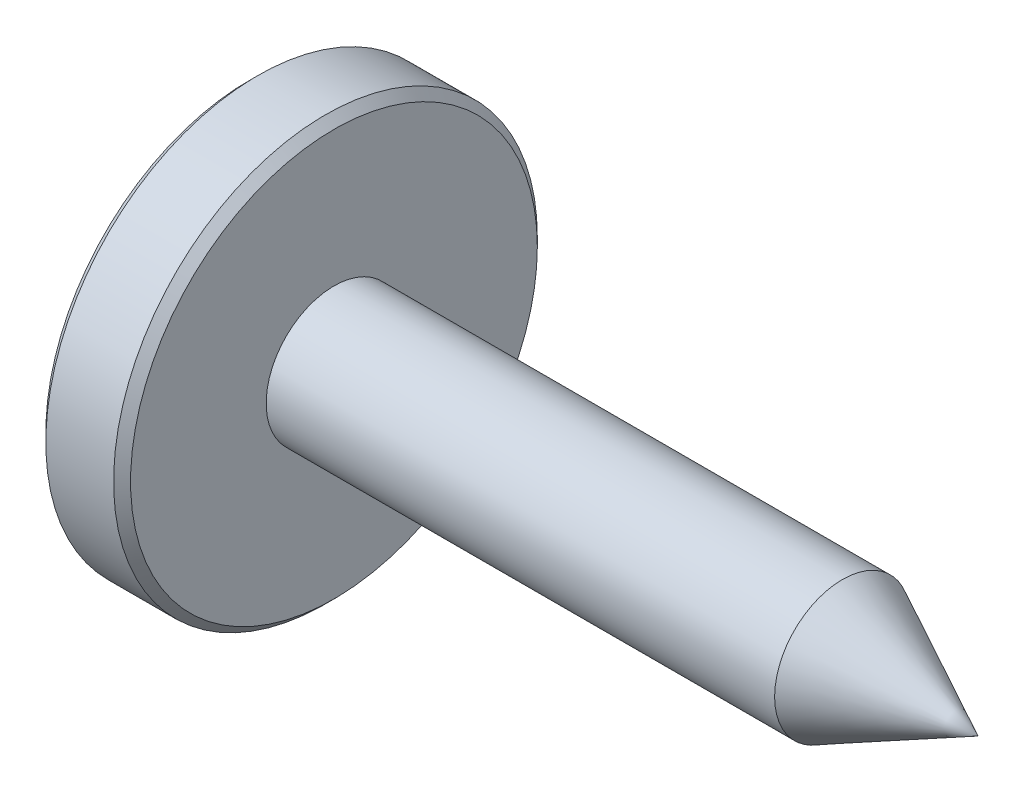
from build123d import *

# Parameters (mm, degrees)
SKETCH_1_R      = 25
EXTRUDE_1_DEPTH = 10
SKETCH_2_R      = 8
EXTRUDE_2_DEPTH = 60
CHAMFER_1_SIZE  = 1


with BuildPart() as part:
    # 草图1 → 凸台-拉伸1 (new body)
    with BuildSketch(Plane(origin=(0, 0, 0), x_dir=(0, 0, -1), z_dir=(1, 0, 0))):
        Circle(SKETCH_1_R)
    extrude(amount=EXTRUDE_1_DEPTH)

    # 草图2 → 凸台-拉伸2 (add)
    with BuildSketch(Plane(origin=(10, 0, 0), x_dir=(0, 0, -1), z_dir=(1, 0, 0))):
        Circle(SKETCH_2_R)
    extrude(amount=EXTRUDE_2_DEPTH)

    # 草图3 → 旋转1 (revolve)
    with BuildSketch(Plane.XY, mode=Mode.PRIVATE) as revolve_1_sk:
        Polygon((70, 8), (86, 0), (70, 0), align=None)
    revolve(revolve_1_sk.sketch.rotate(Axis((0, 0, 0), (1, 0, 0)), 90), axis=Axis((0, 0, 0), (1, 0, 0)))

    # 倒角1
    chamfer_1_edges = [part.edges().sort_by_distance(p)[0] for p in [
        (0, 0, 25),
        (10, 0, 25),
    ]]
    chamfer(chamfer_1_edges, length=CHAMFER_1_SIZE)


solid = part.part
